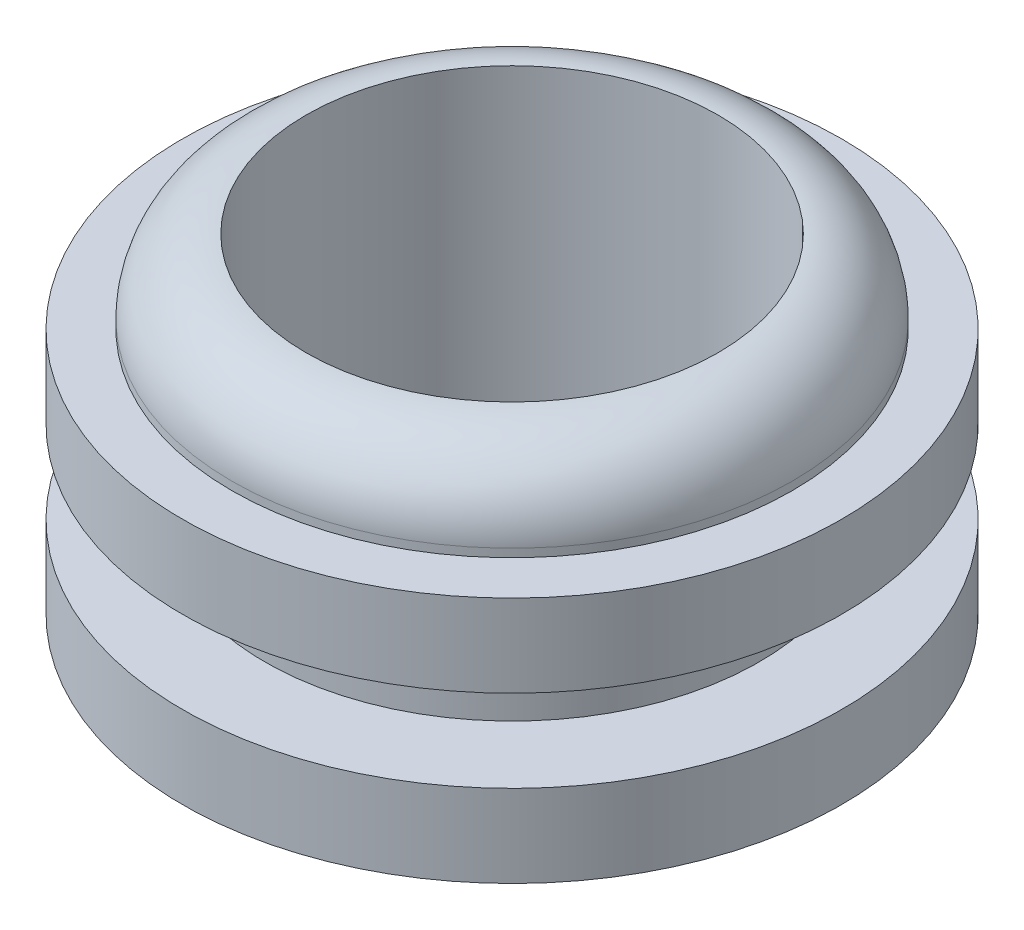
SolidWorks part; units mm, degrees
ref_plane "前视基准面" through (0, 0, 0) normal (0, 0, 1) x (1, 0, 0)
ref_plane "上视基准面" through (0, 0, 0) normal (0, 1, 0) x (1, 0, 0)
ref_plane "右视基准面" through (0, 0, 0) normal (1, 0, 0) x (0, 0, -1)
other "Configuration Table"
sketch "草图1" plane through (0, 0, 0) normal (0, 0, 1) x (1, 0, 0)
  line L0 (0, 0) -> (0, 29.4587) construction
  line L1 (2.5, 0) -> (4, 0)
  line L2 (4, 0) -> (4, 1)
  line L3 (4, 1) -> (3, 1)
  line L4 (3, 1) -> (3, 2)
  line L5 (3, 2) -> (4, 2)
  line L6 (4, 2) -> (4, 3)
  line L7 (4, 3) -> (3.4, 3)
  line L8 (3.4, 3) -> (3.4, 3.1)
  line L10 (2.5, 4) -> (2.5, 0)
  arc A0 (3.4, 3.1) -> (2.5, 4) centre (2.5, 3.1) ccw
  point P16 (3.4, 4)
  dimension "D9" = 0.9
  dimension "D1" = 4
  dimension "D2" = 1
  dimension "D3" = 1
  dimension "D4" = 1
  dimension "D5" = 1
  dimension "D6" = 1
  dimension "D7" = 0
  dimension "D8" = 0.6
  dimension "D10" = 2.5
revolve "旋转1" add sketch "草图1" angle 360 about L0
